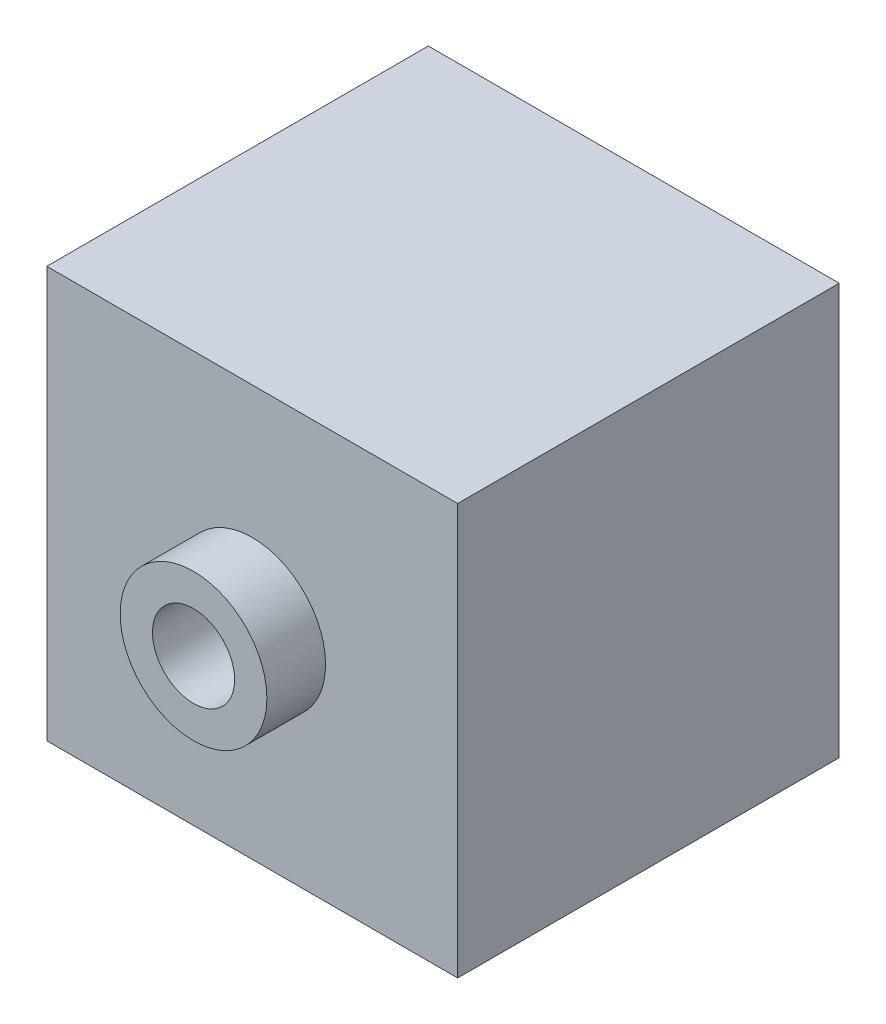
SolidWorks part; units mm, degrees
material "Q235A"
ref_plane "Front Plane" through (0, 0, 0) normal (0, 0, 1) x (1, 0, 0)
ref_plane "Top Plane" through (0, 0, 0) normal (0, 1, 0) x (1, 0, 0)
ref_plane "Right Plane" through (0, 0, 0) normal (1, 0, 0) x (0, 0, -1)
sketch "Sketch1" plane through (0, 0, 0) normal (0, 0, 1) x (1, 0, 0)
  line L1 (35, -35) -> (-35, -35)
  line L2 (35, -35) -> (35, 35)
  line L3 (35, 35) -> (-35, 35)
  line L4 (-35, -35) -> (-35, 35)
  line L5 (35, -35) -> (-35, 35) construction
  line L6 (35, 35) -> (-35, -35) construction
  point P0 (0, 0)
  dimension "D1" = 70
extrude "Boss-Extrude1" add sketch "Sketch1" along normal blind 65
sketch "Sketch2" plane through (0, 0, 65) normal (0, 0, 1) x (1, 0, 0)
  circle A0 centre (0, 0) radius 12.5
  dimension "D1" = 25
extrude "Boss-Extrude2" add sketch "Sketch2" along normal blind 10
hole_wizard "M16 Tapped Hole1" positions "Sketch3" profile "Sketch4" tap size "M16" standard "GB"
sketch "Sketch3" plane through (0, 0, 75) normal (0, 0, 1) x (1, 0, 0)
  point P0 (0, 0)
sketch "Sketch4" plane through (0, 0, 75) normal (1, 0, 0) x (0, -1, 0)
  line L0 (0, 0) -> (0, 46.206)
  line L1 (0, 46.206) -> (7, 42)
  line L2 (7, 42) -> (7, 0)
  line L5 (7, 0) -> (0, 0)
  line L10 (0, 46.206) -> (-7, 42) construction
  line L11 (0, -6.35) -> (0, 107.95) construction
  dimension "螺纹孔钻头直径" = 14
  dimension "螺纹孔钻头深度" = 42
  dimension "导头角度" = 118
cosmetic thread "Hole thread1"
